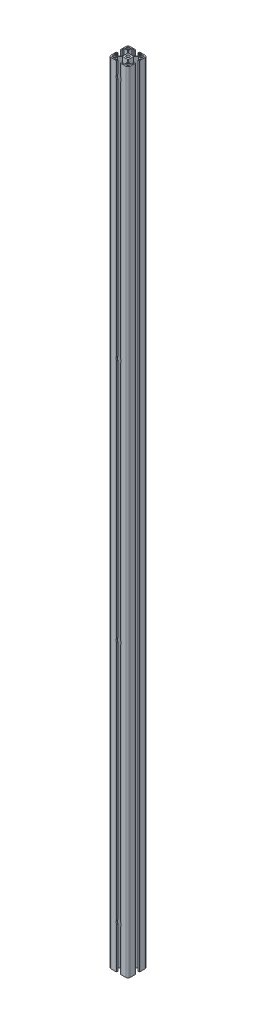
SolidWorks part; units mm, degrees
ref_plane "前视基准面" through (0, 0, 0) normal (0, 0, 1) x (1, 0, 0)
ref_plane "上视基准面" through (0, 0, 0) normal (0, 1, 0) x (1, 0, 0)
ref_plane "右视基准面" through (0, 0, 0) normal (1, 0, 0) x (0, 0, -1)
sketch "草图1" plane through (0, 0, 0) normal (1, 0, 0) x (0, 0, -1)
  line L0 (0, 0) -> (0, 1650)
  dimension "D1" = 1650
other "铝型材 40 X 40L X R4.5(1)"
ref_plane "基准面1" through (0, 0, 0) normal (0, 1, 0) x (0, 0, 1)
sketch "Sketch1" plane through (0, 0, 0) normal (0, 1, 0) x (0, 0, 1)
  line L0 (-5.1, 20) -> (-5.1, 19.5)
  line L1 (-5.1, 19.5) -> (-4.1, 19.5)
  line L2 (-4.1, 19.5) -> (-4.1, 17)
  line L3 (-6.1, 18.5) -> (-10.3, 18.5)
  line L4 (-15.5, -20) -> (-5.1, -20)
  line L5 (-20, -15.5) -> (-20, -5.1)
  line L6 (15.5, 20) -> (5.1, 20)
  line L7 (20, 15.5) -> (20, 5.1)
  line L8 (0, 14.8756) -> (0, 0) construction
  line L9 (0, 0) -> (14.1675, 0) construction
  line L10 (-10.3, 18.5) -> (-10.3, 11.3)
  line L11 (-10.3, 11.3) -> (-5, 6)
  line L12 (-5, 6) -> (5, 6)
  line L13 (10.3, 11.3) -> (5, 6)
  line L14 (10.3, 18.5) -> (10.3, 11.3)
  line L15 (6.1, 18.5) -> (10.3, 18.5)
  line L16 (4.1, 19.5) -> (4.1, 17)
  line L17 (5.1, 19.5) -> (4.1, 19.5)
  line L18 (5.1, 20) -> (5.1, 19.5)
  line L19 (-5.1, 20) -> (-15.5, 20)
  line L20 (20, 5.1) -> (19.5, 5.1)
  line L21 (11.8, 17.5) -> (15, 17.5)
  line L22 (11.8, 17.5) -> (11.8, 11.8)
  line L23 (11.8, 11.8) -> (17.5, 11.8)
  line L24 (17.5, 15) -> (17.5, 11.8)
  line L25 (19.5, 5.1) -> (19.5, 4.1)
  line L26 (19.5, 4.1) -> (17, 4.1)
  line L27 (17, 6.1) -> (17, 4.1)
  line L28 (18.5, 6.1) -> (17, 6.1)
  line L29 (18.5, 6.1) -> (18.5, 10.3)
  line L30 (18.5, 10.3) -> (11.3, 10.3)
  line L31 (11.3, 10.3) -> (6, 5)
  line L32 (6, 5) -> (6, -5)
  line L33 (11.3, -10.3) -> (6, -5)
  line L34 (18.5, -10.3) -> (11.3, -10.3)
  line L35 (18.5, -6.1) -> (18.5, -10.3)
  line L36 (18.5, -6.1) -> (17, -6.1)
  line L37 (17, -4.1) -> (17, -6.1)
  line L38 (19.5, -4.1) -> (17, -4.1)
  line L39 (19.5, -5.1) -> (19.5, -4.1)
  line L40 (20, -5.1) -> (19.5, -5.1)
  line L41 (5.1, -20) -> (5.1, -19.5)
  line L42 (5.1, -19.5) -> (4.1, -19.5)
  line L43 (4.1, -19.5) -> (4.1, -17)
  line L44 (6.1, -17) -> (4.1, -17)
  line L45 (6.1, -18.5) -> (6.1, -17)
  line L46 (6.1, -18.5) -> (10.3, -18.5)
  line L47 (10.3, -18.5) -> (10.3, -11.3)
  line L48 (10.3, -11.3) -> (5, -6)
  line L49 (5, -6) -> (-5, -6)
  line L50 (-10.3, -11.3) -> (-5, -6)
  line L51 (-10.3, -18.5) -> (-10.3, -11.3)
  line L52 (-6.1, -18.5) -> (-10.3, -18.5)
  line L53 (-6.1, -18.5) -> (-6.1, -17)
  line L54 (-4.1, -17) -> (-6.1, -17)
  line L55 (-4.1, -19.5) -> (-4.1, -17)
  line L56 (-5.1, -19.5) -> (-4.1, -19.5)
  line L57 (-5.1, -20) -> (-5.1, -19.5)
  line L58 (-20, -5.1) -> (-19.5, -5.1)
  line L59 (5.1, -20) -> (15.5, -20)
  line L60 (-20, 5.1) -> (-20, 15.5)
  line L61 (-19.5, -5.1) -> (-19.5, -4.1)
  line L62 (-6.1, 18.5) -> (-6.1, 17)
  line L63 (-6.1, 17) -> (-4.1, 17)
  line L64 (6.1, 18.5) -> (6.1, 17)
  line L65 (4.1, 17) -> (6.1, 17)
  line L66 (-19.5, -4.1) -> (-17, -4.1)
  line L67 (-15, 17.5) -> (-11.8, 17.5)
  line L68 (-17.5, 15) -> (-17.5, 11.8)
  line L69 (-17.5, 11.8) -> (-11.8, 11.8)
  line L70 (-11.8, 17.5) -> (-11.8, 11.8)
  line L71 (-17, -6.1) -> (-17, -4.1)
  line L72 (-18.5, -6.1) -> (-17, -6.1)
  line L73 (-18.5, -6.1) -> (-18.5, -10.3)
  line L74 (-18.5, -10.3) -> (-11.3, -10.3)
  line L75 (-11.3, -10.3) -> (-6, -5)
  line L76 (-6, -5) -> (-6, 5)
  line L77 (-11.3, 10.3) -> (-6, 5)
  line L78 (-18.5, 10.3) -> (-11.3, 10.3)
  line L79 (-18.5, 6.1) -> (-18.5, 10.3)
  line L80 (-18.5, 6.1) -> (-17, 6.1)
  line L81 (-17, 4.1) -> (-17, 6.1)
  line L82 (-19.5, 4.1) -> (-17, 4.1)
  line L83 (-19.5, 5.1) -> (-19.5, 4.1)
  line L84 (-20, 5.1) -> (-19.5, 5.1)
  line L85 (20, -5.1) -> (20, -15.5)
  line L87 (-17.5, -11.8) -> (-11.8, -11.8)
  line L88 (-17.5, -11.8) -> (-17.5, -15)
  line L89 (-15, -17.5) -> (-11.8, -17.5)
  line L90 (-11.8, -11.8) -> (-11.8, -17.5)
  line L91 (11.8, -11.8) -> (17.5, -11.8)
  line L92 (11.8, -11.8) -> (11.8, -17.5)
  line L93 (11.8, -17.5) -> (15, -17.5)
  line L94 (17.5, -11.8) -> (17.5, -15)
  circle A0 centre (0, 0) radius 3.4
  arc A1 (-20, 15.5) -> (-15.5, 20) centre (-15.5, 15.5) cw
  arc A2 (20, 15.5) -> (15.5, 20) centre (15.5, 15.5) ccw
  arc A3 (-15.5, -20) -> (-20, -15.5) centre (-15.5, -15.5) cw
  arc A4 (15.5, -20) -> (20, -15.5) centre (15.5, -15.5) ccw
  arc A5 (-15, 17.5) -> (-17.5, 15) centre (-15, 15) ccw
  arc A6 (17.5, 15) -> (15, 17.5) centre (15, 15) ccw
  arc A7 (17.5, -15) -> (15, -17.5) centre (15, -15) cw
  arc A8 (-17.5, -15) -> (-15, -17.5) centre (-15, -15) ccw
  point P2 (0, 10)
  point P4 (0, 0)
  point P5 (-20, -20)
  point P6 (20, -20)
  point P7 (20, 20)
  point P8 (-20, 20)
  point P36 (-20, 20)
  point P39 (20, 20)
  point P121 (0, 0)
  dimension "D1" = 20.6
  dimension "D2" = 40
  dimension "D3" = 8.2
  dimension "D4" = 10.2
  dimension "D5" = 14
  dimension "D6" = 6.8
  dimension "D7" = 4.5
  dimension "D8" = 45
  dimension "D12" = 2.5
  dimension "D13" = 5.7
  dimension "D14" = 1.5
  dimension "D18" = 2.5
  dimension "D19" = 2.5
  dimension "D15" = 2.5
  dimension "D9" = 0.5
  dimension "D10" = 1.5
  dimension "D11" = 10
  dimension "D16" = 3
  dimension "D17" = 2
  dimension "D20" = 1.5
  dimension "D21" = 2.5
hole_wizard "打孔尺寸(%根据)内六角圆柱头螺钉的类型1" positions "草图3" profile "草图4" counterbore size "M6" standard "GB" end condition through all
sketch "草图3" plane through (0, 0, 20) normal (0, 0, 1) x (1, 0, 0)
  line L0 (0, 0) -> (0, 1650) construction
  point P0 (0, 1620)
  dimension "D1" = 30
sketch "草图4" plane through (0, 1620, 20) normal (1, 0, 0) x (0, -1, 0)
  line L0 (0, 0) -> (0, 40)
  line L1 (0, 40) -> (3.3, 40)
  line L3 (3.3, 40) -> (3.3, 6.8)
  line L4 (3.3, 6.8) -> (5.5, 6.8)
  line L5 (5.5, 6.8) -> (5.5, 0)
  line L7 (5.5, 0) -> (0, 0)
  line L11 (0, -6.35) -> (0, 107.95) construction
  dimension "通孔孔直径" = 6.6
  dimension "通孔孔深度" = 40
  dimension "柱形沉头孔直径" = 11
  dimension "柱形沉头孔深度" = 6.8
pattern_linear "阵列(线性)1" count 4 spacing 510 along (0, -1, 0) of "打孔尺寸(%根据)内六角圆柱头螺钉的类型1"
